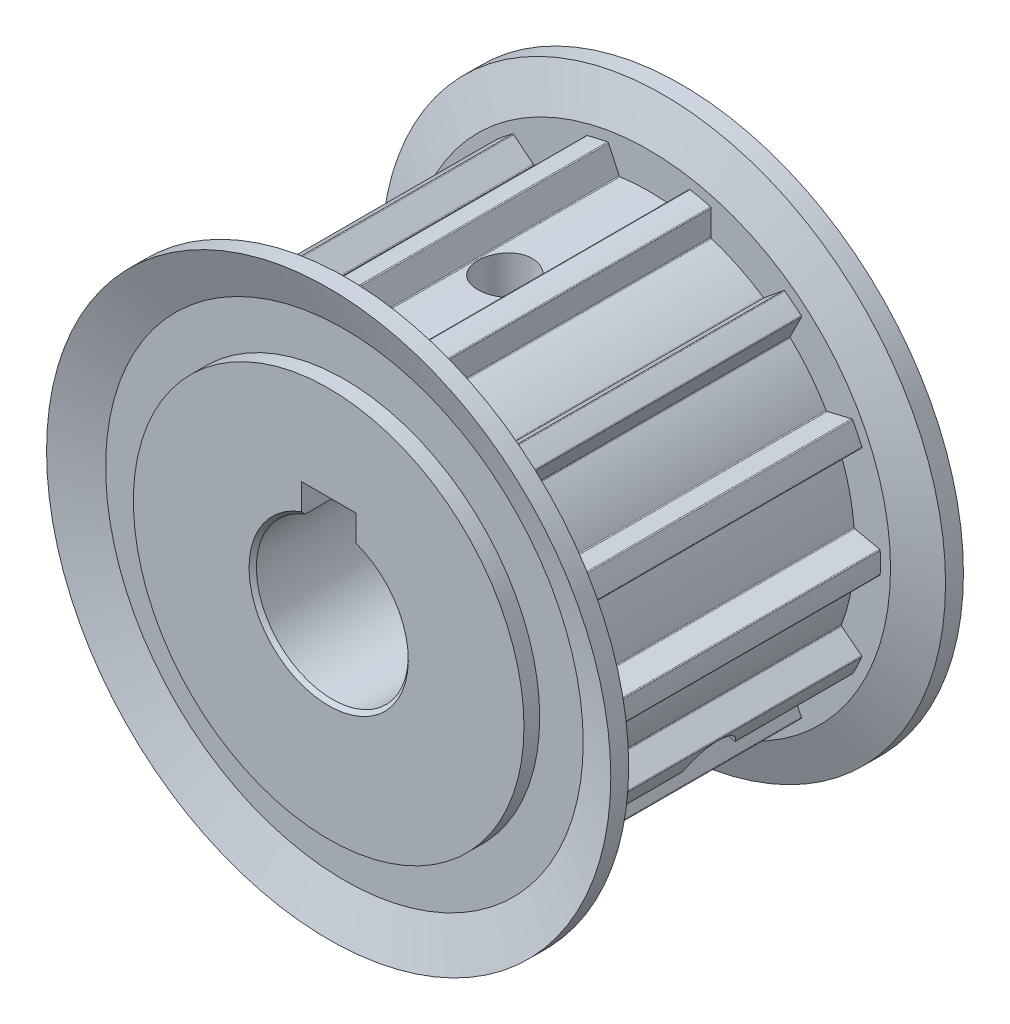
SolidWorks part; units mm, degrees
ref_plane "Front Plane" through (0, 0, 0) normal (0, 0, 1) x (1, 0, 0)
ref_plane "Top Plane" through (0, 0, 0) normal (0, 1, 0) x (1, 0, 0)
ref_plane "Right Plane" through (0, 0, 0) normal (1, 0, 0) x (0, 0, -1)
sketch "Sketch1" plane through (0, 0, 0) normal (1, 0, 0) x (0, 0, -1)
  line L0 (-16.25, 0) -> (16.25, 0) construction
  line L1 (16.25, 0) -> (16.25, 18)
  line L2 (16.25, 18) -> (14.8, 18)
  line L3 (14.8, 18) -> (14.8, 22.0073)
  line L4 (14.8, 22.0073) -> (16.25, 26)
  line L5 (16.25, 26) -> (14.601, 26)
  line L6 (14.601, 26) -> (13.25, 22.28)
  line L7 (13.25, 22.28) -> (13.25, 21.35)
  line L8 (0, 0) -> (0, 26) construction
  line L9 (-31.75, 0) -> (-45.75, 0) construction
  line L10 (-31.75, 0) -> (-16.25, 0) construction
  line L11 (-16.25, 17) -> (-31.75, 17)
  line L12 (-31.75, 17) -> (-31.75, 0)
  line L13 (-26.75, 17) -> (-26.75, 0) construction
  point P10 (13.25, 21.35)
  dimension "D1" = 3
  dimension "W" = 32.5
  dimension "F" = 52
  dimension "D2" = 1.55
  dimension "E" = 36
  dimension "D3" = 1.55
  dimension "PD" = 44.56
  dimension "OD" = 42.7
  dimension "D4" = 5
  dimension "CS" = 14
  dimension "L" = 48
  dimension "D" = 34
sketch "Sketch2" plane through (0, 0, 0) normal (0, 0, 1) x (1, 0, 0)
  line L0 (0, 21.35) -> (0, -21.35) construction
  line L1 (0, 18.99) -> (0, 21.35) construction
  line L3 (2.7363, 18.8635) -> (3.7092, 20.9498)
  line L4 (-2.705, 18.7964) -> (0, 0) construction
  line L5 (0, 0) -> (0, 18.99) construction
  line L6 (0, 0) -> (4.7508, 20.8147) construction
  circle A2 centre (0, 0) radius 18.99 construction
  circle A9 centre (0, 0) radius 21.35 construction
  arc A12 (2.6318, 18.8067) -> (-2.705, 18.7964) centre (0, 0) ccw
  arc A13 (5.7489, 20.5614) -> (3.8177, 21.0059) centre (0, 0) ccw
  arc A14 (2.6318, 18.8067) -> (2.7363, 18.8635) centre (2.6457, 18.9058) ccw
  arc A15 (3.7092, 20.9498) -> (3.8177, 21.0059) centre (3.7998, 20.9075) cw
  point P6 (0, 18.99)
  point P17 (2.705, 18.7964)
  point P20 (3.7417, 21.0196)
  point P29 (0, 21.35)
  dimension "D1" = 2.36
  dimension "D5" = 0.1
  dimension "D6" = 12.857
  dimension "D2" = 5.41
  dimension "D7" = 0.1
  dimension "D3" = 25
sketch "Sketch3" plane through (0, 0, 0) normal (1, 0, 0) x (0, 0, -1)
  line L0 (16.25, 0) -> (16.25, 18) construction
  line L1 (16.25, 18) -> (14.8, 18) construction
  line L2 (14.8, 18) -> (14.8, 22.0073) construction
  line L3 (14.8, 22.0073) -> (16.25, 26) construction
  line L4 (16.25, 26) -> (14.601, 26) construction
  line L5 (14.601, 26) -> (13.25, 22.28) construction
  line L7 (16.25, 0) -> (16.25, 18)
  line L8 (16.25, 18) -> (14.8, 18)
  line L9 (14.8, 18) -> (14.8, 22.0073)
  line L10 (14.8, 22.0073) -> (16.25, 26)
  line L11 (16.25, 26) -> (14.601, 26)
  line L12 (14.601, 26) -> (13.25, 22.28)
  line L13 (13.25, 22.28) -> (13.25, 18.99)
  line L15 (13.25, 18.99) -> (-13.25, 18.99)
  line L16 (0, 0) -> (0, 26) construction
  line L17 (0, 0) -> (0, 26) construction
  line L18 (-13.25, 22.28) -> (-13.25, 18.99)
  line L19 (-14.601, 26) -> (-13.25, 22.28)
  line L20 (-16.25, 26) -> (-14.601, 26)
  line L21 (-14.8, 22.0073) -> (-16.25, 26)
  line L22 (-14.8, 18) -> (-14.8, 22.0073)
  line L23 (-16.25, 18) -> (-14.8, 18)
  line L24 (-16.25, 0) -> (-16.25, 18)
  line L25 (-16.25, 0) -> (16.25, 0)
  point P14 (0, 18.99)
revolve "Revolve1" add sketch "Sketch3" angle 360 about L0
sketch "Sketch4" plane through (0, 0, 0) normal (0, 0, 1) x (1, 0, 0)
  line L1 (0, 0) -> (4.7508, 20.8147) construction
  line L2 (0, 0) -> (4.7508, 20.8147) construction
  line L3 (2.7363, 18.8635) -> (3.7092, 20.9498) construction
  line L4 (2.7363, 18.8635) -> (3.7092, 20.9498)
  line L5 (5.7192, 18.1827) -> (5.7479, 20.4844)
  arc A1 (2.6318, 18.8067) -> (2.7363, 18.8635) centre (2.6457, 18.9058) ccw construction
  arc A3 (3.8177, 21.0059) -> (3.7092, 20.9498) centre (3.7998, 20.9075) ccw construction
  arc A4 (5.7489, 20.5614) -> (3.8177, 21.0059) centre (0, 0) ccw construction
  arc A5 (2.6318, 18.8067) -> (2.7363, 18.8635) centre (2.6457, 18.9058) ccw
  arc A6 (3.8177, 21.0059) -> (3.7092, 20.9498) centre (3.7998, 20.9075) ccw
  arc A7 (5.6745, 20.5821) -> (3.8177, 21.0059) centre (0, 0) ccw
  circle A8 centre (0, 0) radius 18.99 construction
  arc A10 (5.7887, 18.0862) -> (2.6318, 18.8067) centre (0, 0) ccw
  arc A11 (5.7887, 18.0862) -> (5.7192, 18.1827) centre (5.8192, 18.1814) cw
  arc A12 (5.6745, 20.5821) -> (5.7479, 20.4844) centre (5.6479, 20.4857) cw
extrude "Boss-Extrude1" add sketch "Sketch4" along normal mid plane 26.5
pattern_circular "CirPattern1" count 14 over 360 about axis through (0, 0, 0) along (0, 0, 1) of "Boss-Extrude1"
sketch "Sketch14" plane through (0, 0, 0) normal (1, 0, 0) x (0, 0, -1)
  line L0 (-16.25, 26) -> (-16.25, -26) construction
  line L1 (-31.75, 17) -> (-16.25, 17)
  line L2 (-31.75, 17) -> (-31.75, 0)
  line L3 (-31.75, 0) -> (-16.25, 0)
  line L4 (-16.25, 17) -> (-16.25, 0)
revolve "Revolve2" [suppressed] add sketch "Sketch14" angle 360 about L3
sketch "Sketch H" plane through (0, 0, 0) normal (1, 0, 0) x (0, 0, -1)
  line L0 (16.25, 0) -> (16.25, 18) construction
  line L1 (-16.25, 0) -> (16.25, 0) construction
  line L2 (-16.25, 0) -> (16.25, 0) construction
  point P0 (16.25, 0.5)
  dimension "dH" = 1
sketch "Sketch6" [suppressed] plane through (0, 0, 0) normal (0, 0, 1) x (1, 0, 0)
  circle A0 centre (0, 0) radius 17.5
extrude "Cut-Extrude1" [suppressed] cut sketch "Sketch6" against normal through all and the other way through all
chamfer "Chamfer1" [suppressed] distance 0.21 angle 45
sketch "Sketch P" plane through (0, 0, 0) normal (0, 0, 1) x (1, 0, 0)
  line L0 (0, 0) -> (0, 26) construction
  line L1 (0, 0) -> (0, 26) construction
  circle A0 centre (0, 0) radius 0.5
  point P3 (0.25, 0.433)
  dimension "dP" = 1
  dimension "MP" = 0.5
sketch "Sketch19" [suppressed] plane through (0, 0, 0) normal (0, 0, 1) x (1, 0, 0)
  circle A0 centre (0, 0) radius 2.5 construction
  circle A1 centre (0, 0) radius 2.5
extrude "Cut-Extrude5" [suppressed] cut sketch "Sketch19" against normal through all and the other way through all
chamfer "Chamfer6" [suppressed] distance 0.05 angle 45
sketch "Sketch20" [suppressed] plane through (0, 0, 0) normal (0, 1, 0) x (1, 0, 0)
  circle A0 centre (0, 0) radius 1.5
  point P4 (1.5, 0)
extrude "Cut-Extrude6" cut sketch "Sketch20" along normal through all
cosmetic thread "Cosmetic Thread3" [suppressed] parameters "D2"=0.6
ref_plane "Plane2" [suppressed] through (0, 0, 0) normal (-0.866, 0.5, 0) x (-0.5, -0.866, 0)
sketch "Sketch21" [suppressed] plane through (0, 0, 0) normal (-0.866, 0.5, 0) x (-0.5, -0.866, 0)
  circle A0 centre (0, 0) radius 1.5
  dimension "D1" = 0.5
extrude "Cut-Extrude7" cut sketch "Sketch21" against normal through all
cosmetic thread "Cosmetic Thread4" [suppressed] parameters "D2"=0.6
chamfer "Chamfer7" [suppressed] distance 0.035 angle 45
sketch "Sketch N" plane through (0, 0, 0) normal (0, 0, 1) x (1, 0, 0)
  line L0 (-2.5, 6.5383) -> (-2.5, 9.3)
  line L1 (-2.5, 9.3) -> (2.5, 9.3)
  line L2 (2.5, 9.3) -> (2.5, 6.5383)
  line L3 (0, 0) -> (0, 26) construction
  line L4 (0, 0) -> (0, 26) construction
  arc A0 (-2.5, 6.5383) -> (2.5, 6.5383) centre (0, 0) ccw
  point P1 (0, 7)
  point P8 (2.5, 9.3)
  dimension "dN" = 14
  dimension "bN" = 5
  dimension "tN" = 2.3
  dimension "MN" = 5
sketch "Sketch9" plane through (0, 0, 0) normal (0, 0, 1) x (1, 0, 0)
  line L0 (-2.5, 6.5383) -> (-2.5, 9.3) construction
  line L1 (-2.5, 9.3) -> (2.5, 9.3) construction
  line L2 (2.5, 9.3) -> (2.5, 6.5383) construction
  line L3 (-2.5, 6.5383) -> (-2.5, 9.3)
  line L4 (-2.5, 9.3) -> (2.5, 9.3)
  line L5 (2.5, 9.3) -> (2.5, 6.5383)
  arc A0 (-2.5, 6.5383) -> (2.5, 6.5383) centre (0, 0) ccw construction
  arc A1 (-2.5, 6.5383) -> (2.5, 6.5383) centre (0, 0) ccw
extrude "Cut-Extrude2" cut sketch "Sketch9" against normal through all and the other way through all
chamfer "Chamfer2" distance 0.34 angle 45 2 edges at (0, -7, -16.25) (0, -7, 16.25)
sketch "Sketch15" plane through (0, 0, 0) normal (0, 1, 0) x (1, 0, 0)
  circle A0 centre (0, 0) radius 2.5
  point P2 (2.5, 0)
extrude "Cut-Extrude3" cut sketch "Sketch15" along normal through all from vertex at 9.3 starting at point (2.5, 9.3, 0)
cosmetic thread "Cosmetic Thread1" parameters "D2"=5.1
ref_plane "Plane1" through (0, 0, 0) normal (-0.866, 0.5, 0) x (-0.5, -0.866, 0)
sketch "Sketch16" plane through (0, 0, 0) normal (-0.866, 0.5, 0) x (-0.5, -0.866, 0)
  circle A0 centre (0, 0) radius 2.5
  dimension "D1" = 5
extrude "Cut-Extrude4" cut sketch "Sketch16" against normal through all
cosmetic thread "Cosmetic Thread2" parameters "D2"=5.1
chamfer "Chamfer5" [suppressed] distance 0.25 angle 45
sketch "Sketch V" plane through (0, 0, 0) normal (1, 0, 0) x (0, 0, -1)
  line L0 (-16.25, 0.5) -> (14.25, 0.5)
  line L1 (14.25, 0.5) -> (14.25, 1.5)
  line L2 (14.25, 1.5) -> (16.25, 1.5)
  line L3 (-16.25, 0) -> (16.25, 0) construction
  line L4 (-16.25, 0) -> (16.25, 0) construction
  dimension "dV" = 1
  dimension "ZV" = 3
  dimension "JV" = 2
sketch "Sketch11" [suppressed] plane through (0, 0, 0) normal (1, 0, 0) x (0, 0, -1)
  line L1 (1.5, 4) -> (1.5, 5) construction
  line L2 (1.5, 5) -> (5.5, 5) construction
  line L3 (-5.5, 4) -> (1.5, 4)
  line L4 (1.5, 4) -> (1.5, 5)
  line L5 (1.5, 5) -> (5.5, 5)
  line L6 (-5.5, 4) -> (-5.5, 0)
  line L7 (-5.5, 0) -> (5.5, 0)
  line L8 (5.5, 0) -> (5.5, 5)
revolve "Cut-Revolve1" [suppressed] cut sketch "Sketch11" angle 360 about L0
chamfer "Chamfer3" [suppressed] distance 0.13 angle 45
sketch "Sketch F" plane through (0, 0, 0) normal (1, 0, 0) x (0, 0, -1)
  line L0 (-16.25, 0) -> (16.25, 0) construction
  line L3 (-16.25, 0) -> (16.25, 0) construction
  line L4 (-16.25, 0) -> (-16.25, 5)
  line L5 (-16.25, 26) -> (-16.25, -26) construction
  line L8 (-16.25, 5) -> (-12.25, 5)
  line L9 (-12.25, 5) -> (-12.25, 4)
  line L10 (-12.25, 4) -> (16.25, 4)
  line L11 (16.25, 4) -> (16.25, 0)
  dimension "ZF" = 10
  dimension "dF" = 8
  dimension "JF" = 4
sketch "Sketch22" [suppressed] plane through (0, 0, 0) normal (1, 0, 0) x (0, 0, -1)
  line L0 (-11.5, 0) -> (-11.5, 5)
  line L2 (-11.5, 7) -> (-11.5, 0) construction
  line L3 (-11.5, 5) -> (-7.5, 5)
  line L4 (-5, 5) -> (-1, 5) construction
  line L6 (-7.5, 5) -> (-7.5, 4)
  line L9 (5, 4) -> (5, 0)
  line L10 (5, 0) -> (-11.5, 0)
  line L11 (-7.5, 4) -> (5, 4)
revolve "Cut-Revolve3" [suppressed] cut sketch "Sketch22" angle 360 about L10
chamfer "Chamfer8" [suppressed] distance 0.18 angle 45
sketch "Sketch Y" plane through (0, 0, 0) normal (1, 0, 0) x (0, 0, -1)
  line L2 (-16.25, 0) -> (16.25, 0) construction
  line L3 (-16.25, 0) -> (16.25, 0) construction
  line L4 (-16.25, 0.05) -> (-13.25, 0.05)
  line L5 (-13.25, 0.05) -> (-13.25, 1.5)
  line L6 (-13.25, 1.5) -> (13.25, 1.5)
  line L7 (13.25, 1.5) -> (13.25, 0.05)
  line L8 (13.25, 0.05) -> (16.25, 0.05)
  dimension "dY" = 3
  dimension "QY" = 0.1
  dimension "RY" = 0.1
  dimension "SY" = 3
  dimension "TY" = 3
sketch "Sketch13" [suppressed] plane through (0, 0, 0) normal (1, 0, 0) x (0, 0, -1)
  line L0 (-5.5, 4) -> (-2.5, 4) construction
  line L1 (-2.5, 4) -> (-2.5, 2.5) construction
  line L2 (-2.5, 2.5) -> (2.5, 2.5) construction
  line L3 (2.5, 2.5) -> (2.5, 4.5) construction
  line L4 (2.5, 4.5) -> (5.5, 4.5) construction
  line L5 (-5.5, 4) -> (-2.5, 4)
  line L6 (-2.5, 4) -> (-2.5, 2.5)
  line L7 (-2.5, 2.5) -> (2.5, 2.5)
  line L8 (2.5, 2.5) -> (2.5, 4.5)
  line L9 (2.5, 4.5) -> (5.5, 4.5)
  line L10 (-5.5, 4) -> (-5.5, 0)
  line L11 (-5.5, 0) -> (5.5, 0)
  line L12 (5.5, 0) -> (5.5, 4.5)
revolve "Cut-Revolve2" [suppressed] cut sketch "Sketch13" angle 360 about L0
chamfer "Chamfer4" [suppressed] distance 0.02 angle 45
sketch "Sketch23" [suppressed] plane through (0, 0, 0) normal (0, 0, 1) x (1, 0, 0)
  line L0 (0, 5) -> (0, 0) construction
  line L1 (-2, 6.8) -> (2, 6.8)
  line L2 (-2, 6.8) -> (-2, 4.5826)
  line L4 (2, 6.8) -> (2, 4.5826)
  arc A0 (-2, 4.5826) -> (2, 4.5826) centre (0, 0) ccw
  circle A2 centre (0, 0) radius 5 construction
  dimension "D1" = 10
  dimension "D2" = 4
  dimension "D3" = 1.8
extrude "Cut-Extrude8" [suppressed] cut sketch "Sketch23" against normal through all and the other way through all
chamfer "Chamfer9" [suppressed] distance 0.3 angle 45
sketch "Sketch24" [suppressed] plane through (0, 0, 0) normal (0, 1, 0) x (1, 0, 0)
  circle A0 centre (0, 0) radius 2
  dimension "D1" = 4
extrude "Cut-Extrude9" cut sketch "Sketch24" along normal through all
cosmetic thread "Cosmetic Thread5" [suppressed] parameters "D2"=4.1
pattern_circular "CirPattern2" [suppressed] count 2 over 120
